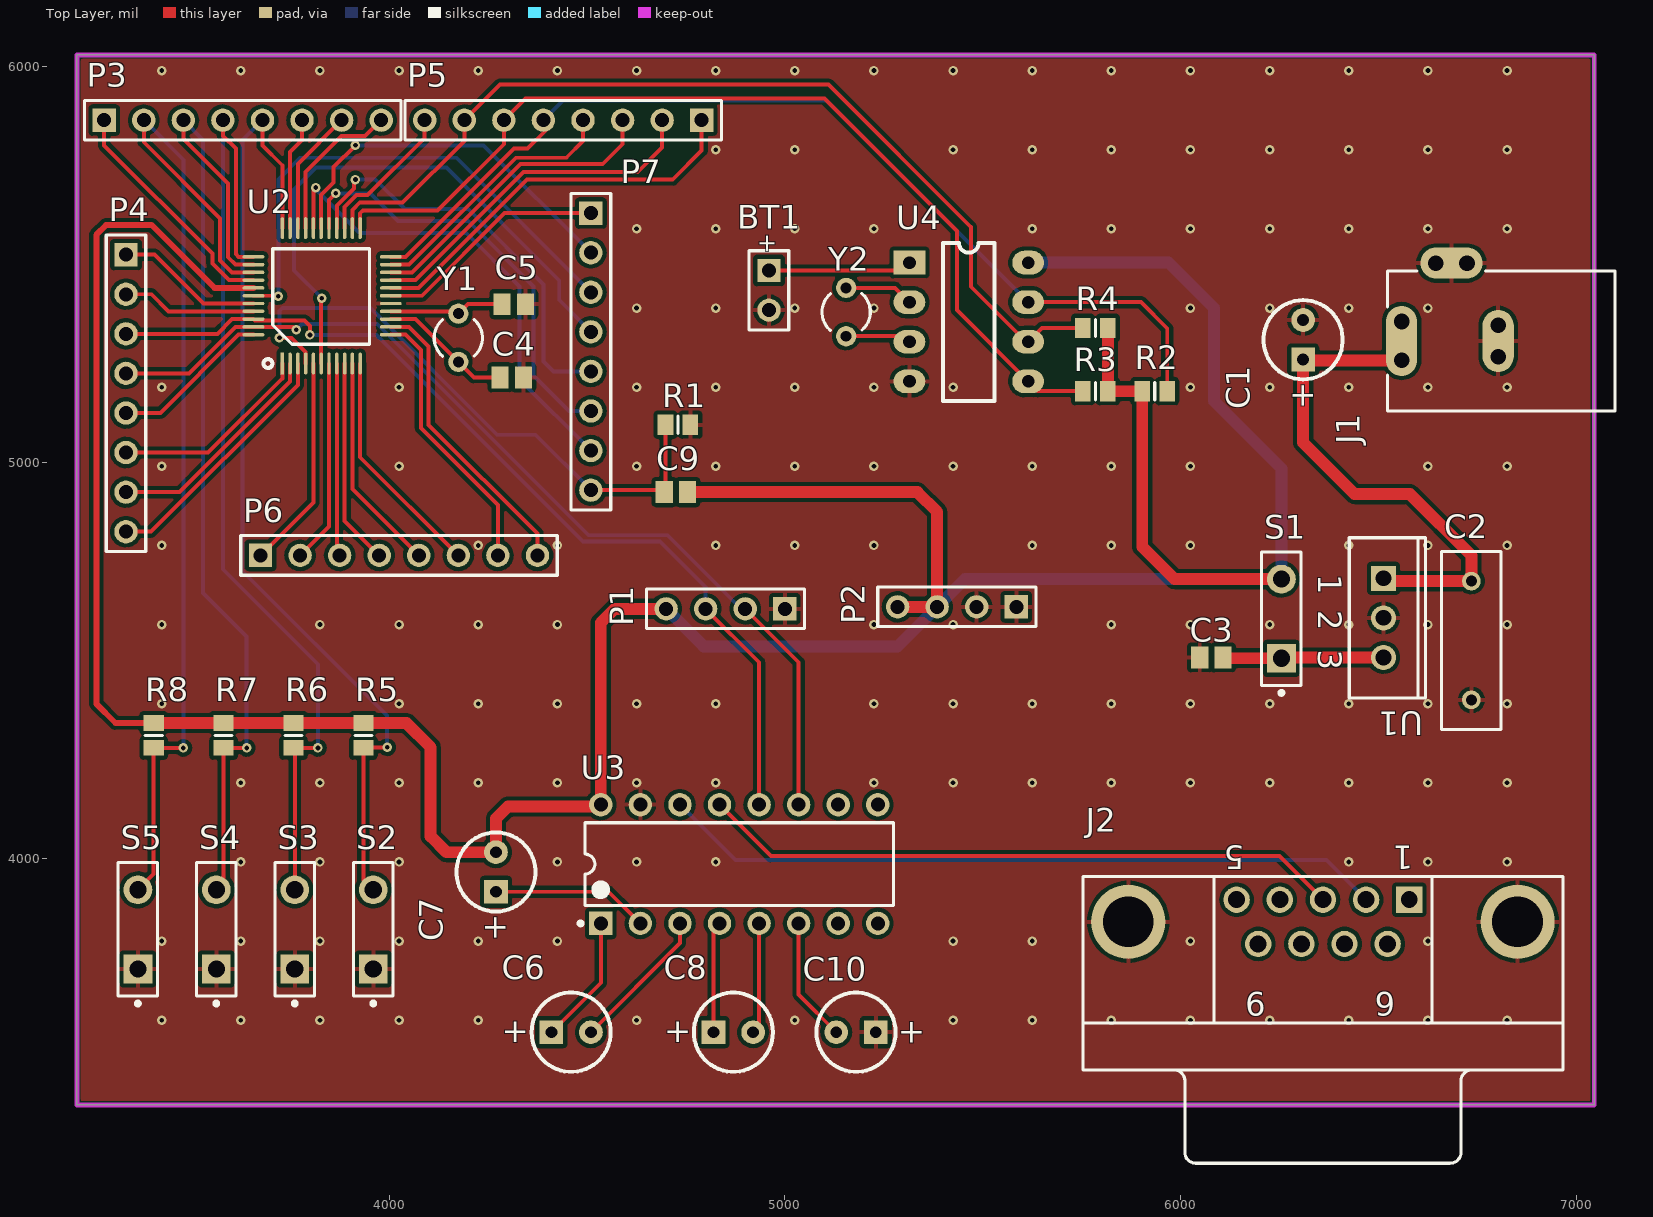
[diagram p0: Top Layer view]
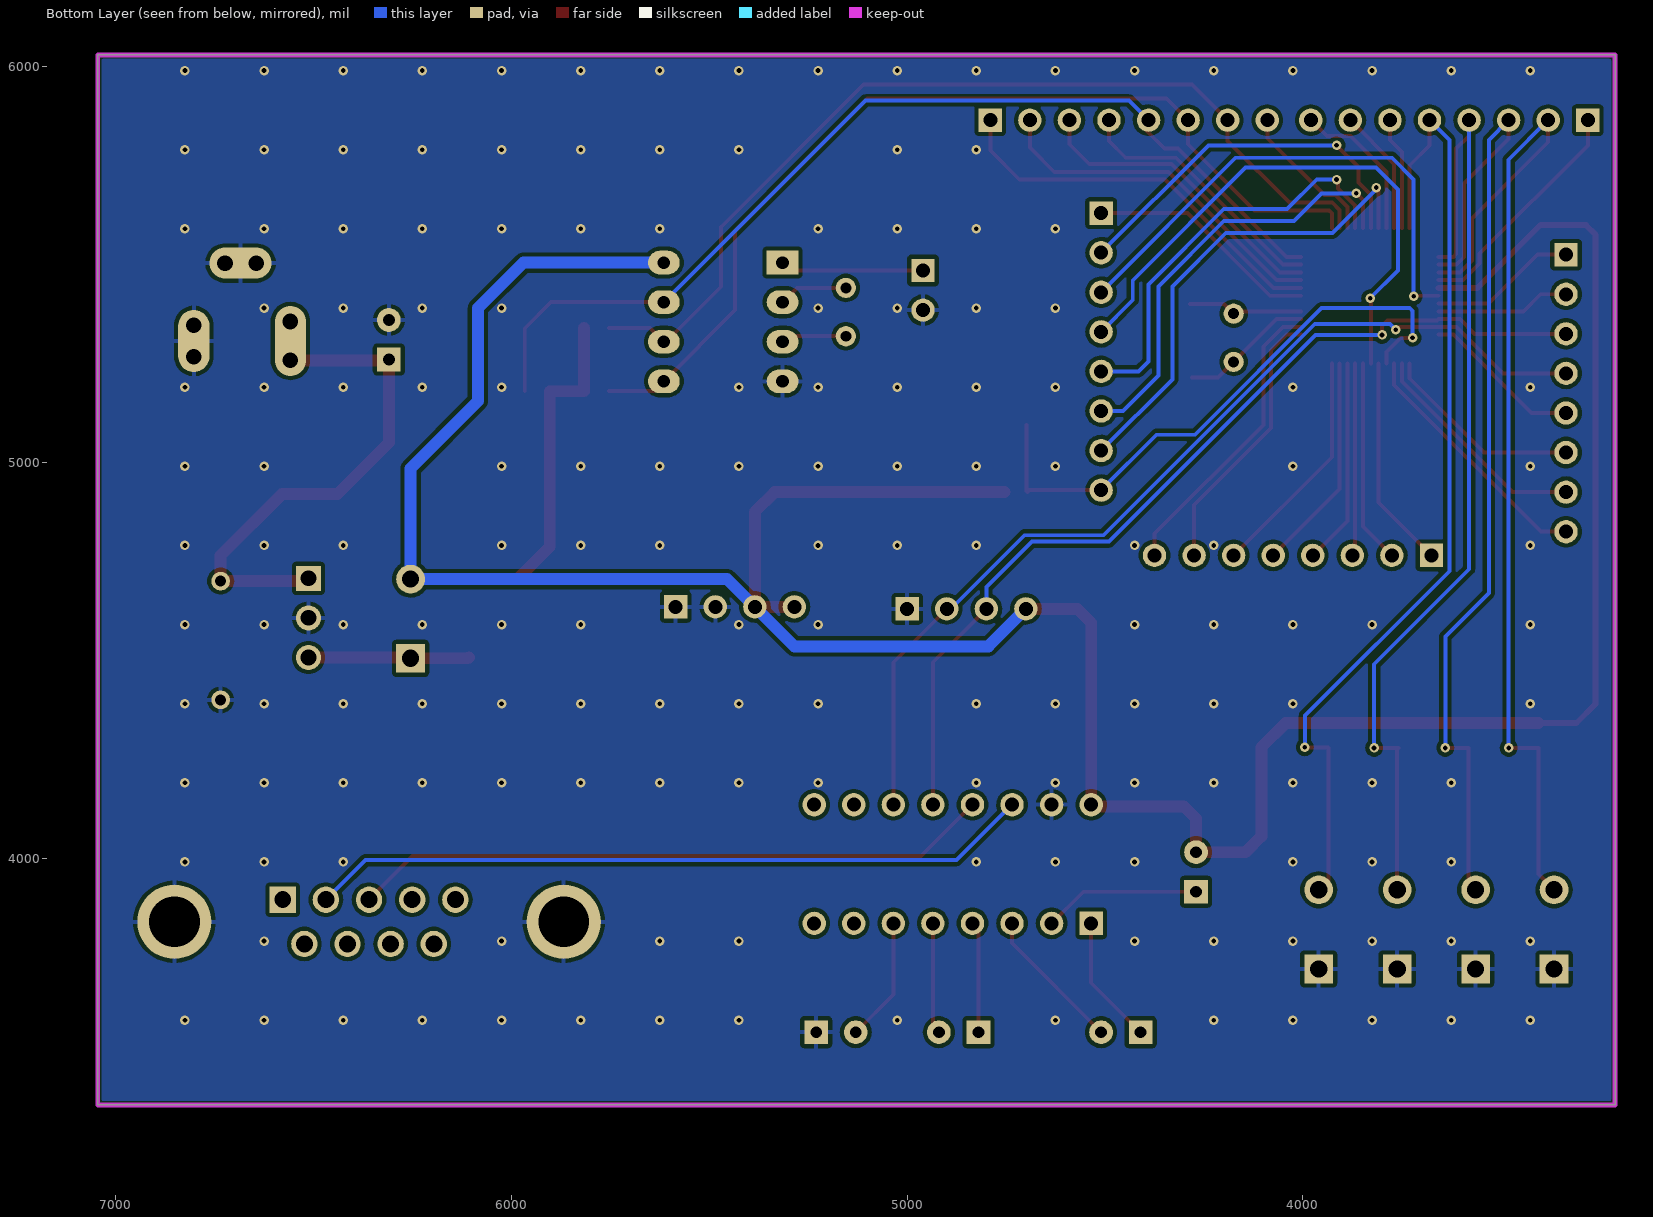
[diagram p1: Bottom Layer view, seen from below]
# Altium PCB MISC50994.pcbdoc
Units mil, origin at the board's own origin, x right, y up, seen from the top; angles counter-clockwise.
Board outline 3834.65 x 2653.54 mil, 2 copper layers (Top Layer, Bottom Layer), stack 40.6 mil thick; 39 components, 57 nets, 191 pads, 174 vias.

## Layer stack, top to bottom
Top Solder Mask Layer: solder mask 0.4, Solder Resist, Dk 3.5
Top Layer: signal copper 1.4
SUBSTRATE1: surface 12.6, FR-4, Dk 4.8
SUBSTRATE2: surface 12.6, FR-4, Dk 4.8
SUBSTRATE3: surface 12.6, FR-4, Dk 4.8
Bottom Layer: signal copper 1.4
Bottom Solder Mask Layer: solder mask 0.4, Solder Resist, Dk 3.5

## Board outline
7045.83,3376.18 3211.18,3376.18 3211.18,6029.72 7045.83,6029.72

## Design rules (kind name [scope] priority, off if disabled: settings)
BoardOutlineClearance Plane_innerPlane_1 [All] p2 off: genericclearance=6 ignorepadtopadclearanceinfootprint=FALSE except(0: Arc-SplitContinuation Track-SplitContinuation SMDPad-SplitContinuation THPad-SplitContinuation Via-SplitContinuation Fill-SplitContinuation Region-SplitContinuation Poly-SplitContinuation Text-SplitContinuation Hole-SplitContinuation; 6: Arc-CutoutEdge Track-CutoutEdge SMDPad-CutoutEdge THPad-CutoutEdge Via-CutoutEdge Fill-CutoutEdge Region-CutoutEdge Text-CutoutEdge; 6.9: Hole-OutlineEdge Hole-CutoutEdge; 10: Poly-OutlineEdge Poly-CutoutEdge; 11.8: Arc-OutlineEdge Track-OutlineEdge SMDPad-OutlineEdge THPad-OutlineEdge Via-OutlineEdge Fill-OutlineEdge Region-OutlineEdge Text-OutlineEdge)
BoardOutlineClearance Copper_copperRegion_1 [All] p4 off: genericclearance=6 ignorepadtopadclearanceinfootprint=FALSE except(0: Arc-SplitContinuation Track-SplitContinuation SMDPad-SplitContinuation THPad-SplitContinuation Via-SplitContinuation Fill-SplitContinuation Region-SplitContinuation Poly-SplitContinuation Text-SplitContinuation Hole-SplitContinuation; 6: Arc-CutoutEdge Track-CutoutEdge SMDPad-CutoutEdge THPad-CutoutEdge Via-CutoutEdge Fill-CutoutEdge Region-CutoutEdge Text-CutoutEdge; 6.9: Hole-OutlineEdge Hole-CutoutEdge; 10: Poly-OutlineEdge Poly-CutoutEdge; 11.8: Arc-OutlineEdge Track-OutlineEdge SMDPad-OutlineEdge THPad-OutlineEdge Via-OutlineEdge Fill-OutlineEdge Region-OutlineEdge Text-OutlineEdge)
BoardOutlineClearance safeClearance_1 [All] p6: genericclearance=6 ignorepadtopadclearanceinfootprint=FALSE except(0: Arc-SplitContinuation Track-SplitContinuation SMDPad-SplitContinuation THPad-SplitContinuation Via-SplitContinuation Fill-SplitContinuation Region-SplitContinuation Poly-SplitContinuation Text-SplitContinuation Hole-SplitContinuation; 6: Arc-CutoutEdge Track-CutoutEdge SMDPad-CutoutEdge THPad-CutoutEdge Via-CutoutEdge Fill-CutoutEdge Region-CutoutEdge Text-CutoutEdge; 6.9: Hole-OutlineEdge Hole-CutoutEdge; 10: Poly-OutlineEdge Poly-CutoutEdge; 11.8: Arc-OutlineEdge Track-OutlineEdge SMDPad-OutlineEdge THPad-OutlineEdge Via-OutlineEdge Fill-OutlineEdge Region-OutlineEdge Text-OutlineEdge)
Clearance Plane_innerPlane [All] p1 off: gap=6 ignorepadtopadclearanceinfootprint=FALSE except(6.9: Hole-Track Hole-SMDPad Hole-THPad Hole-Via Fill-Hole Region-Hole Hole-Arc Hole-Text; 10: Poly-Track Poly-SMDPad Poly-THPad Poly-Via Poly-Fill Poly-Region Poly-Poly Poly-Arc Poly-Text Poly-Hole)
Clearance Copper_copperRegion [All] p3 off: gap=6 ignorepadtopadclearanceinfootprint=FALSE except(6.9: Hole-Track Hole-SMDPad Hole-THPad Hole-Via Fill-Hole Region-Hole Hole-Arc Hole-Text; 10: Poly-Track Poly-SMDPad Poly-THPad Poly-Via Poly-Fill Poly-Region Poly-Poly Poly-Arc Poly-Text Poly-Hole)
Clearance safeClearance [All] p5: gap=6 ignorepadtopadclearanceinfootprint=FALSE except(6.9: Hole-Track Hole-SMDPad Hole-THPad Hole-Via Fill-Hole Region-Hole Hole-Arc Hole-Text; 10: Poly-Track Poly-SMDPad Poly-THPad Poly-Via Poly-Fill Poly-Region Poly-Poly Poly-Arc Poly-Text Poly-Hole)
DiffPairsRouting differentialPair [All] p1: maxlimit=6 minlimit=6 mostfreqgap=6 toplayer_minwidth=5 toplayer_prefwidth=10 toplayer_maxwidth=100 toplayer_mingap=6 toplayer_prefgap=6 toplayer_maxgap=6 bottomlayer_minwidth=5 bottomlayer_prefwidth=10 bottomlayer_maxwidth=100 bottomlayer_mingap=6 bottomlayer_prefgap=6 bottomlayer_maxgap=6 maxuncoupledlength=10
Length netLength [All] p1: minlimit=0 maxlimit=0
PasteMaskExpansion pasteMaskExpansion [All] p1: expansion=0
PlaneConnect innerPlane [All] p1: planeconnectstyle=Relief reliefexpansion=20 reliefentries=4 reliefconductorwidth=10 reliefairgap=10
PolygonConnect copperRegion [All] p1: connectstyle=Relief reliefconductorwidth=10 reliefentries=4 polygonreliefangle="90 Angle" airgapwidth=10 via.connectstyle=Relief via.reliefconductorwidth=10 via.reliefentries=4 via.polygonreliefangle="90 Angle" via.airgapwidth=10
RoutingVias viaSize [All] p1: holewidth=12.01 width=24.02 viastyle="Through Hole" minholewidth=11.81 minwidth=19.68 maxholewidth=236.22 maxwidth=393.7
SolderMaskExpansion solderMaskExpansion [IsVia] p1: expansion=-1000 istentingtop=TRUE
SolderMaskExpansion solderMaskExpansion [All] p2: expansion=2 istentingtop=FALSE
Width trackWidth [All] p1: maxlimit=100 minlimit=5 preferedwidth=10
1 further rules are at their usual default settings.

## Components (designator, comment, footprint, x,y, rotation, side; value= is the part's Value field where it differs from the comment)
BT1 "Battery" BAT-2 4960,5435 r270 top
C1 "Cap Pol1" RB2.54-5.08 6310,5260 r90 top
C2 "Cap" RAD-0.3 6735,4550 r90 top
C3 "Cap" C0805 6078.15,4506.95 r0 top
C4 "Cap" C0805 4310,5215 r0 top
C5 "Cap" C0805 4315,5400 r0 top
C6 "Cap Pol1" RB2.54-5.08 4410,3560 r0 top
C7 "Cap Pol1" RB2.54-5.08 4270,3915 r90 top
C8 "Cap Pol1" RB2.54-5.08 4820,3560 r0 top
C9 "Cap" C0805 4725,4925 r0 top
C10 "Cap Pol1" RB2.54-5.08 5230,3560 r180 top
J1 "PWR2.5" KLD-0202 7098.15,5306.95 r180 top
J2 "D Connector 9" DSUB1.385-2H9 6360,3465 r180 top
P1 "DEBUG" HDR1X4 5000,4630 r180 top
P2 "POWER" HDR1X4 5585,4635 r180 top
P3 "PIN0" HDR1X8 3280,5865 r0 top
P4 "PIN1" HDR1X8 3335,5525 r270 top
P5 "PIN2" HDR1X8 4790,5865 r180 top
P6 "PIN3" HDR1X8 3675,4765 r0 top
P7 "PIN4" HDR1X8 4510,5630 r270 top
R1 "Res2" 6-0805_L 4730,5095 r180 top
R2 "Res2" 6-0805_L 5935,5180 r180 top
R3 "Res2" 6-0805_L 5785,5180 r0 top
R4 "Res2" 6-0805_L 5785,5340 r180 top
R5 "Res2" 6-0805_L 3935,4310 r90 top
R6 "Res2" 6-0805_L 3758.33,4310 r90 top
R7 "Res2" 6-0805_L 3581.67,4310 r90 top
R8 "Res2" 6-0805_L 3405,4310 r90 top
S1 "SW-SPST" SPST-2 6255,4605 r90 top
S2 "SW-PB" SPST-2 3960,3820 r90 top
S3 "SW-PB" SPST-2 3761.67,3820 r90 top
S4 "SW-PB" SPST-2 3563.33,3820 r90 top
S5 "SW-PB" SPST-2 3365,3820 r90 top
U1 "MC7805BT" 221A-04 6513.15,4606.95 r270 top
U2 "STC12C5A60S2" TQFP-44 3730,5250 r0 top
U3 "MAX232ACPE" PE16A 4885,3985 r90 top
U4 "DS1302" DIP-8 5315,5505 r0 top
Y1 "XTAL" R38 4175,5315 r0 top
Y2 "XTAL" R38 5155,5380 r180 top

## Footprints (in the part's own frame and the unit in brackets; to place one, negate y for a bottom-side part, rotate by r counter-clockwise, add the part's x,y. Pads: shape width x height; smd on the part's side, far side on the other; paste and mask are expansions set on the pad)
6-0805_L [mm]
  rect 1x1.3 smd: 1(-0.8,0) 2(0.8,0)
  silkscreen extent 0,-0.55 0,0.55
221A-04 [mm]
  rect 1.6x1.6 hole 1: 1(-2.54,0)
  round 1.6 hole 1: 2(0,0) 3(2.54,0)
  silkscreen extent -5.15,-2.2 5.15,2.7
BAT-2 [mm]
  rect 1.5x1.5 hole 0.9: 1(-1.27,0)
  round 1.5 hole 0.9: 2(1.27,0)
  silkscreen extent -2.54,-1.27 2.54,1.27
C0805 [mm]
  rect 1.1x1.4 smd: 1(-0.75,0) 2(0.75,0)
DIP-8 [mil]
  rect 80x60 hole 32: 1(0,0)
  oval 80x60 hole 32: 2(0,-100) 3(0,-200) 4(0,-300) 5(300,-300) 6(300,-200) 7(300,-100) 8(300,0)
  silkscreen extent 85,-350 215,50
DSUB1.385-2H9 [mm]
  rect 1.69x1.69 hole 1.09: 1(-5.54,-10.92)
  round 1.69 hole 1.09: 2(-2.77,-10.92) 3(0,-10.92) 4(2.77,-10.92) 5(5.54,-10.92) 6(-4.155,-8.08) 7(-1.385,-8.08) 8(1.385,-8.08) 9(4.155,-8.08)
  round 4.76 hole 3.26: 10(-12.495,-9.5) 11(12.495,-9.5)
  silkscreen extent -15.4,-12.4 15.4,6
HDR1X4 [mm]
  rect 1.5x1.5 hole 0.9: 1(0,0)
  round 1.5 hole 0.9: 2(2.54,0) 3(5.08,0) 4(7.62,0)
  silkscreen extent -1.27,-1.27 8.89,1.27
HDR1X8 [mm]
  rect 1.5x1.5 hole 0.9: 1(0,0)
  round 1.5 hole 0.9: 2(2.54,0) 3(5.08,0) 4(7.62,0) 5(10.16,0) 6(12.7,0) 7(15.24,0) 8(17.78,0)
  silkscreen extent -1.27,-1.27 19.05,1.27
KLD-0202 [mm]
  oval 2x4.5 all layers, no hole: 1(13.7,0)
  round 1.5 hole 1: 1A(13.7,-1.25) 1B(13.7,1.25) 2A(7.5,-1) 2B(7.5,1) 3A(9.5,-5) 3B(11.5,-5)
  oval 2x4 all layers, no hole: 2(7.5,0)
  oval 4x2 all layers, no hole: 3(10.5,-5)
  silkscreen extent 0,-4.5 14.6,4.5
PE16A [mm]
  rect 1.5x1.5 hole 0.9: 1(-3.81,8.89)
  round 1.5 hole 0.9: 2(-3.81,6.35) 3(-3.81,3.81) 4(-3.81,1.27) 5(-3.81,-1.27) 6(-3.81,-3.81) 7(-3.81,-6.35) 8(-3.81,-8.89) 9(3.81,-8.89) 10(3.81,-6.35) 11(3.81,-3.81) 12(3.81,-1.27) 13(3.81,1.27) 14(3.81,3.81) 15(3.81,6.35) 16(3.81,8.89)
  silkscreen extent -3.93,-9.9 2.65,10.31
R38 [mm]
  round 1.3 hole 0.7: 1(0,1.55) 2(0,-1.55)
  silkscreen extent -1.55,-1.19 1.55,1.17
RAD-0.3 [mm]
  round 1.2 hole 0.7: 1(-3.81,0) 2(3.81,0)
  silkscreen extent -5.71,-1.91 5.71,1.91
RB2.54-5.08 [mil]
  rect 60x60 hole 30: 1(0,0)
  round 60 hole 30: 2(100,0)
  silkscreen extent -50,-100 150,100
SPST-2 [mm]
  rect 1.85x1.85 hole 1.1: 1(-2.54,0)
  round 1.85 hole 1.1: 2(2.54,0)
  silkscreen extent -4.89,-1.27 4.28,1.27
TQFP-44 [mm]
  rect 0.22x1.4 smd: 1(0,0)
  oval 0.22x1.4 smd: 2(0.5,0) 3(1,0) 4(1.5,0) 5(2,0) 6(2.5,0) 7(3,0) 8(3.5,0) 9(4,0) 10(4.5,0) 11(5,0) 23(5,8.692) 24(4.5,8.692) 25(4,8.692) 26(3.5,8.692) 27(3,8.692) 28(2.5,8.692) 29(2,8.692) 30(1.5,8.692) 31(1,8.692) 32(0.5,8.692) 33(0,8.692)
  oval 1.4x0.22 smd: 12(6.969,1.85) 13(6.969,2.35) 14(6.969,2.85) 15(6.969,3.35) 16(6.969,3.85) 17(6.969,4.35) 18(6.969,4.85) 19(6.969,5.35) 20(6.969,5.85) 21(6.969,6.35) 22(6.969,6.85) 34(-1.85,6.85) 35(-1.85,6.35) 36(-1.85,5.85) 37(-1.85,5.35) 38(-1.85,4.85) 39(-1.85,4.35) 40(-1.85,3.85) 41(-1.85,3.35) 42(-1.85,2.85) 43(-1.85,2.35) 44(-1.85,1.85)
  silkscreen extent -1.2,-0.28 5.59,7.37

## Via types
v1: diameter 24.02, hole 12, Top Layer to Bottom Layer, 161 vias
v2: diameter 24, hole 12, Top Layer to Bottom Layer, 13 vias

## Nets (pads, with @x,y where several pads share a name; then routed paths per layer and width w, separated by ;. In a path a pad name is that pad's centre, name@x,y a point inside that pad or via, vN(x,y) a via of type N, cw(c..) or ccw(c..) an arc to the next point about the centre after c; other vN are vias at no path point)
GND: BT1.2 C1.2 C2.1 C3.1 C4.2 C5.2 C10.1 J1.2 J1.2A J1.2B J1.3 J1.3A J1.3B J2.10 J2.11 P1.1 P2.1 P2.2 R1.1 S2.1 S3.1 S4.1 S5.1 U1.2 U2.16 U3.15 U4.4
  other v1: 3425.28,3590.28 3625.28,3590.28 3825.28,3590.28 4025.28,3590.28 4225.28,3590.28 4625.28,3590.28 5025.28,3590.28 5425.28,3590.28 5625.28,3590.28 5825.28,3590.28 6025.28,3590.28 6225.28,3590.28 6425.28,3590.28 6625.28,3590.28 6825.28,3590.28 3425.28,3790.28 3625.28,3790.28 3825.28,3790.28 4025.28,3790.28 4225.28,3790.28 4425.28,3790.28 5425.28,3790.28 5625.28,3790.28 6025.28,3790.28 6625.28,3790.28 3625.28,3990.28 3825.28,3990.28 4025.28,3990.28 4425.28,3990.28 4625.28,3990.28 4825.28,3990.28 6425.28,3990.28 6625.28,3990.28 6825.28,3990.28 3625.28,4190.28 3825.28,4190.28 4025.28,4190.28 4225.28,4190.28 4425.28,4190.28 4625.28,4190.28 4825.28,4190.28 5225.28,4190.28 5425.28,4190.28 5625.28,4190.28 5825.28,4190.28 6025.28,4190.28 6225.28,4190.28 6425.28,4190.28 6625.28,4190.28 6825.28,4190.28 3425.28,4390.28 4025.28,4390.28 4225.28,4390.28 4425.28,4390.28 4625.28,4390.28 4825.28,4390.28 5225.28,4390.28 5425.28,4390.28 5625.28,4390.28 5825.28,4390.28 6025.28,4390.28 6225.28,4390.28 6425.28,4390.28 6625.28,4390.28 6825.28,4390.28 3425.28,4590.28 3825.28,4590.28 4025.28,4590.28 4225.28,4590.28 4425.28,4590.28 5225.28,4590.28 5425.28,4590.28 5825.28,4590.28 6025.28,4590.28 6225.28,4590.28 6425.28,4590.28 6625.28,4590.28 6825.28,4590.28 3425.28,4790.28 4225.28,4790.28 4425.28,4790.28 4825.28,4790.28 5025.28,4790.28 5225.28,4790.28 5625.28,4790.28 5825.28,4790.28 6025.28,4790.28 6425.28,4790.28 6625.28,4790.28 6825.28,4790.28 3425.28,4990.28 4025.28,4990.28 4625.28,4990.28 4825.28,4990.28 5025.28,4990.28 5225.28,4990.28 5425.28,4990.28 5625.28,4990.28 5825.28,4990.28 6025.28,4990.28 6625.28,4990.28 6825.28,4990.28 3425.28,5190.28 4025.28,5190.28 4625.28,5190.28 4825.28,5190.28 5025.28,5190.28 5225.28,5190.28 5425.28,5190.28 6025.28,5190.28 6225.28,5190.28 6425.28,5190.28 6625.28,5190.28 6825.28,5190.28 4625.28,5390.28 4825.28,5390.28 5025.28,5390.28 5225.28,5390.28 6025.28,5390.28 6225.28,5390.28 6425.28,5390.28 6625.28,5390.28 4625.28,5590.28 4825.28,5590.28 5025.28,5590.28 5225.28,5590.28 5625.28,5590.28 5825.28,5590.28 6025.28,5590.28 6225.28,5590.28 6425.28,5590.28 6625.28,5590.28 6825.28,5590.28 4825.28,5790.28 5025.28,5790.28 5425.28,5790.28 5625.28,5790.28 5825.28,5790.28 6025.28,5790.28 6225.28,5790.28 6425.28,5790.28 6625.28,5790.28 6825.28,5790.28 3425.28,5990.28 3625.28,5990.28 3825.28,5990.28 4025.28,5990.28 4225.28,5990.28 4425.28,5990.28 4625.28,5990.28 4825.28,5990.28 5025.28,5990.28 5225.28,5990.28 5425.28,5990.28 5625.28,5990.28 5825.28,5990.28 6025.28,5990.28 6225.28,5990.28 6425.28,5990.28 6625.28,5990.28 6825.28,5990.28
NETBT1_1: BT1.1 U4.1 | length 363.3
  Top Layer w10: BT1.1 5295,5485 U4.1
NETC1_1: C1.1 C2.2 J1.1 J1.1A J1.1B U1.1 | length 1292.5
  Top Layer w30: U1.1 6520.1,4700 C2.2 6735,4765 6580,4920 6440,4920 6310,5050 C1.1 6312.26,5257.74 J1.1B
NETC3_2: C3.2 S1.1 U1.3 | length 407.1
  Top Layer w30: C3.2 6109.63,4505 S1.1 6256.95,4506.95 U1.3
NETC6_1: C6.1 U3.1 | length 326.8
  Top Layer w10: C6.1 4535,3685 U3.1
NETC6_2: C6.2 U3.3 | length 368.2
  Top Layer w10: C6.2 4735,3785 U3.3
NETC7_1: C7.1 U3.2 | length 398.1
  Top Layer w10: C7.1 4555,3915 U3.2
NETC8_1: C8.1 U3.4 | length 281.2
  Top Layer w10: C8.1 4820,3820 U3.4
NETC8_2: C8.2 U3.5 | length 281.2
  Top Layer w10: C8.2 4935,3575 U3.5
NETC10_2: C10.2 U3.6 | length 314.4
  Top Layer w10: U3.6 5035,3655 C10.2
NETJ2_2: J2.2 U3.14 | length 1833.5
  Bottom Layer w10: U3.14 4875,3995 6368.98,3995 J2.2
NETJ2_3: J2.3 U3.13 | length 1624.4
  Top Layer w10: U3.13 4965,4005 6249.92,4005 J2.3
NETU4_2: U4.2 Y2.2 | length 174.9
  Top Layer w10: Y2.2 5278.98,5441.02 U4.2
NETU4_3: U4.3 Y2.1 | length 165.8
  Top Layer w10: Y2.1 5301.02,5318.98 U4.3
P0_0: P3.1 U2.37 | length 596.9
  Top Layer w10: P3.1 3280,5801.01 3553.48,5527.53 3553.48,5502.29 3595.14,5460.63 U2.37
P0_1: P3.2 R8.1 S5.2 U2.36 | length 2609
  Top Layer w10: S5.2 3405,3960 R8.1 v2(3480,4278.5) ; P3.2 3380,5809.16 3573.16,5616 3573.16,5510.45 3603.3,5480.31 U2.36
  Bottom Layer w10: P3.2 3480,5765 v2(3480,4278.5)
P0_2: P3.3 R7.1 S4.2 U2.35 | length 2542.4
  Top Layer w10: P3.3 3480,5817.32 3592.85,5704.47 3592.85,5518.6 3611.45,5500 U2.35 ; S4.2 3581.67,3938.33 R7.1 v2(3640,4278.5)
  Bottom Layer w10: P3.3 3530,5815 3530,4670 3640,4560 v2(3640,4278.5)
P0_3: P3.4 R6.1 S3.2 U2.34 | length 2506.7
  Top Layer w10: P3.4 3580,5825.47 3612.53,5792.94 3612.53,5526.76 3619.61,5519.69 U2.34 ; S3.2 3761.67,4275.17 R6.1 v2(3820,4278.5)
  Bottom Layer w10: P3.4 3580,4730 3820,4490 v2(3820,4278.5)
P0_4: P3.5 R5.1 S2.2 U2.33 | length 2479.9
  Top Layer w10: P3.5 3680,5801.01 3730,5751.01 U2.33 ; S2.2 3935,3945 R5.1 3936.5,4280 v2(3995,4280)
  Bottom Layer w10: P3.5 3630,5815 3630,4725 3995,4360 v2(3995,4280)
P0_5: P3.6 U2.32 | length 285.4
  Top Layer w10: U2.32 3749.68,5784.69 3780,5815 P3.6
P0_6: P3.7 U2.31 | length 318.6
  Top Layer w10: U2.31 3769.37,5754.37 P3.7
P0_7: P3.8 U2.30 | length 387
  Top Layer w10: U2.30 3789.05,5734.06 3879.47,5824.47 3939.47,5824.47 P3.8
P1_0: P4.1 U2.40 | length 373.3
  Top Layer w10: P4.1 3407.14,5525 3530.57,5401.57 U2.40
P1_1: P4.2 U2.41 | length 340
  Top Layer w10: P4.2 3398.99,5425 3442.1,5381.89 U2.41
P1_2: P1.3 P4.3 U2.42 U3.12 | length 2380.2
  Top Layer w10: P4.3 3566.09,5325 3603.3,5362.2 U2.42 3660.85,5358.52 3786.48,5358.52 3800,5345 v2(3800,5322.2) ; P1.3 4935,4495 U3.12
  Bottom Layer w10: v2(3800,5322.2) 3967.8,5322.2 4490,4800 4685,4800 4800,4685 P1.3
P1_3: P1.2 P4.4 U2.43 U3.11 | length 2471.7
  Top Layer w10: P4.4 3493.93,5225 3611.45,5342.52 U2.43 3758.49,5342.52 v2(3765.49,5335.52) ; P1.2 5035,4495 U3.11
  Bottom Layer w10: v2(3765.49,5335.52) 3779.97,5350 3970,5350 4504,4816 4704,4816 4890,4630 P1.2
P1_4: P4.5 U2.44 | length 404.1
  Top Layer w10: P4.5 3421.77,5125 3619.61,5322.84 U2.44
P1_5: P4.6 U2.1 | length 510.2
  Top Layer w10: P4.6 3542.56,5025 3730,5212.44 U2.1
P1_6: P4.7 U2.2 | length 576.1
  Top Layer w10: P4.7 3470.4,4925 3749.68,5204.29 U2.2
P1_7: P4.8 U2.3 | length 642
  Top Layer w10: P4.8 3398.24,4825 3769.37,5196.13 U2.3
P2_0: P5.1 U2.18 | length 1006.5
  Top Layer w10: U2.18 4074.54,5440.94 4348.28,5714.69 4716.83,5714.69 4790,5787.86 P5.1
P2_1: P5.2 U2.19 | length 893.5
  Top Layer w10: U2.19 4066.39,5460.63 4340.13,5734.37 4628.36,5734.37 4690,5796.01 P5.2
P2_2: P5.3 U2.20 | length 780.6
  Top Layer w10: U2.20 4058.24,5480.31 4331.98,5754.06 4539.89,5754.06 4590,5804.16 P5.3
P2_3: P5.4 U2.21 | length 667.7
  Top Layer w10: U2.21 4050.08,5500 4320.14,5770.06 4447.74,5770.06 4490,5812.32 P5.4
P2_4: P5.5 R2.1 U2.22 U4.7 | length 2547.1
  Top Layer w10: U2.22 4041.93,5519.69 4315.67,5793.43 4350.27,5793.43 4396.35,5839.5 4396.35,5858.65 P5.5 ; U4.7 5900,5405 5966.5,5338.5 R2.1
  Bottom Layer w10: P5.5 4440,5915 5105,5915 U4.7
P2_5: P5.6 R3.1 U2.23 U4.5 | length 2443.7
  Top Layer w10: U2.23 3926.85,5629.76 3933.92,5636.83 4122.67,5636.83 4290,5804.16 P5.6 4345,5920 5100,5920 5435,5585 5435,5385 U4.5 5640,5180 R3.1
P2_6: P5.7 R4.2 U2.24 U4.6 | length 2425.9
  Top Layer w10: U2.24 3907.16,5637.92 3925.77,5656.52 4034.2,5656.52 4190,5812.32 P5.7 4280,5955 5110,5955 5470,5595 5470,5445 5610,5305 U4.6 5650,5340 R4.2
P2_7: P5.8 U2.25 | length 373.2
  Top Layer w10: U2.25 3887.48,5646.07 3917.61,5676.2 3945.73,5676.2 4090,5820.47 P5.8
P3_0: P6.1 U2.5 | length 540.4
  Top Layer w10: P6.1 3808.74,4898.74 U2.5
P3_1: P6.2 U2.7 | length 515.3
  Top Layer w10: P6.2 3848.11,4838.11 U2.7
P3_2: P6.3 U2.8 | length 488
  Top Layer w10: U2.8 3867.8,4772.2 P6.3
P3_3: P6.4 U2.9 | length 521.3
  Top Layer w10: U2.9 3887.48,4852.52 P6.4
P3_4: P6.5 U2.10 | length 554.5
  Top Layer w10: U2.10 3907.16,4932.84 P6.5
P3_5: P6.6 U2.11 | length 587.8
  Top Layer w10: U2.11 3926.85,5013.15 P6.6
P3_6: P6.7 U2.12 | length 691.9
  Top Layer w10: U2.12 4041.93,5322.84 4080.32,5284.45 4080.32,5086.85 4275,4892.16 P6.7
P3_7: P6.8 U2.13 | length 757.8
  Top Layer w10: U2.13 4050.08,5342.52 4100,5292.6 4100,5095 4375,4820 P6.8
P4_0: P7.1 U2.17 | length 592.1
  Top Layer w10: U2.17 4082.7,5421.26 4291.44,5630 P7.1
P4_1: P7.2 U2.28 | length 952.6
  Top Layer w10: U2.28 3828.43,5675.95 3860,5707.53 3860,5746.47 v2(3915,5801.47)
  Bottom Layer w10: v2(3915,5801.47) 4238.53,5801.47 P7.2
P4_2: P7.3 U2.39 | length 1312
  Top Layer w10: U2.39 3718.74,5421.26 v2(3720,5420)
  Bottom Layer w10: v2(3720,5420) 3720,5715 3775,5770 4170,5770 P7.3
P4_3: P7.4 U2.6 | length 1443.6
  Top Layer w10: U2.6 3828.43,5413.43 v2(3830,5415)
  Bottom Layer w10: v2(3830,5415) 3760,5485 3760,5690 3815,5745 4145,5745 4430,5460 4430,5410 P7.4
P4_4: P7.5 U2.26 | length 1052.5
  Top Layer w10: U2.26 3867.8,5649.01 3910.99,5692.2 3910.99,5710.99 v2(3915,5715)
  Bottom Layer w10: v2(3915,5715) 3965,5715 4040,5640 4200,5640 4390,5450 4390,5255 4415,5230 P7.5
P4_5: P7.6 U2.27 | length 1099.4
  Top Layer w10: U2.27 3848.11,5663.11 v2(3865,5680)
  Bottom Layer w10: v2(3865,5680) 3952.97,5680 4022.97,5610 4200,5610 4365,5445 4365,5220 4455,5130 P7.6
P4_6: P7.7 U2.29 | length 1215.5
  Top Layer w10: U2.29 3808.74,5688.79 v2(3814.5,5694.56)
  Bottom Layer w10: v2(3814.5,5694.56) 3814.5,5690.5 3925,5580 4195,5580 4330,5445 4330,5210 P7.7
P4_7: C9.1 P7.8 R1.2 U2.4 | length 1517.6
  Top Layer w10: v2(3722.93,5315) 3753.55,5315 3789.05,5279.5 U2.4 ; P7.8 4690.47,4930 C9.1 4698.5,4928.03 R1.2
  Bottom Layer w10: v2(3722.93,5315) 3722.93,5382.93 3730,5390 3952.63,5390 4272.63,5070 4370,5070 P7.8
VCC: C7.2 C9.2 P1.4 P2.3 P2.4 R2.2 R3.2 R4.1 R5.2 R6.2 R7.2 R8.2 S1.2 U2.38 U3.16 U4.8 | length 8914.3
  Top Layer w15: R8.2 3308.5,4341.5 3260,4390 3260,5575 3285,5600 3400,5600 3559.05,5440.94 U2.38
  Top Layer w30: R8.2 R7.2 R6.2 R5.2 4043.5,4341.5 4105,4280 4105,4055 4145,4015 C7.2 4270,4100 4300,4130 4530,4130 U3.16 4535,4595 4570,4630 P1.4 ; C9.2 5335,4925 5385,4875 P2.3 P2.4 ; R4.1 R3.2 R2.2 5903.5,4786.5 5985,4705 S1.2
  Bottom Layer w30: P1.4 4795,4535 5285,4535 P2.3 5455,4705 S1.2 6255,4985 6085,5155 6085,5390 5970,5505 U4.8
XTAL1: C5.1 U2.15 Y1.1 | length 293.5
  Top Layer w10: U2.15 4169.13,5381.89 Y1.1 4198.98,5400 C5.1
XTAL2: C4.1 U2.14 Y1.2 | length 337.1
  Top Layer w10: U2.14 4066.77,5362.2 Y1.2 4213.98,5215 C4.1
pads on no net: J2.1 J2.4 J2.5 J2.6 J2.7 J2.8 J2.9 U3.7 U3.8 U3.9 U3.10

## Polygon pours and split planes (outlines as drawn)
GND on Top Layer (solid, remove dead copper, pour order 0): 3000,6290 3000,3000 7675,3000 7675,6290
GND on Bottom Layer (solid, remove dead copper, pour order 2): 3020,6160 3020,3185 7350,3185 7350,6160

## Keep-outs
Board Outline Layer:
  the board outline again, w11.81